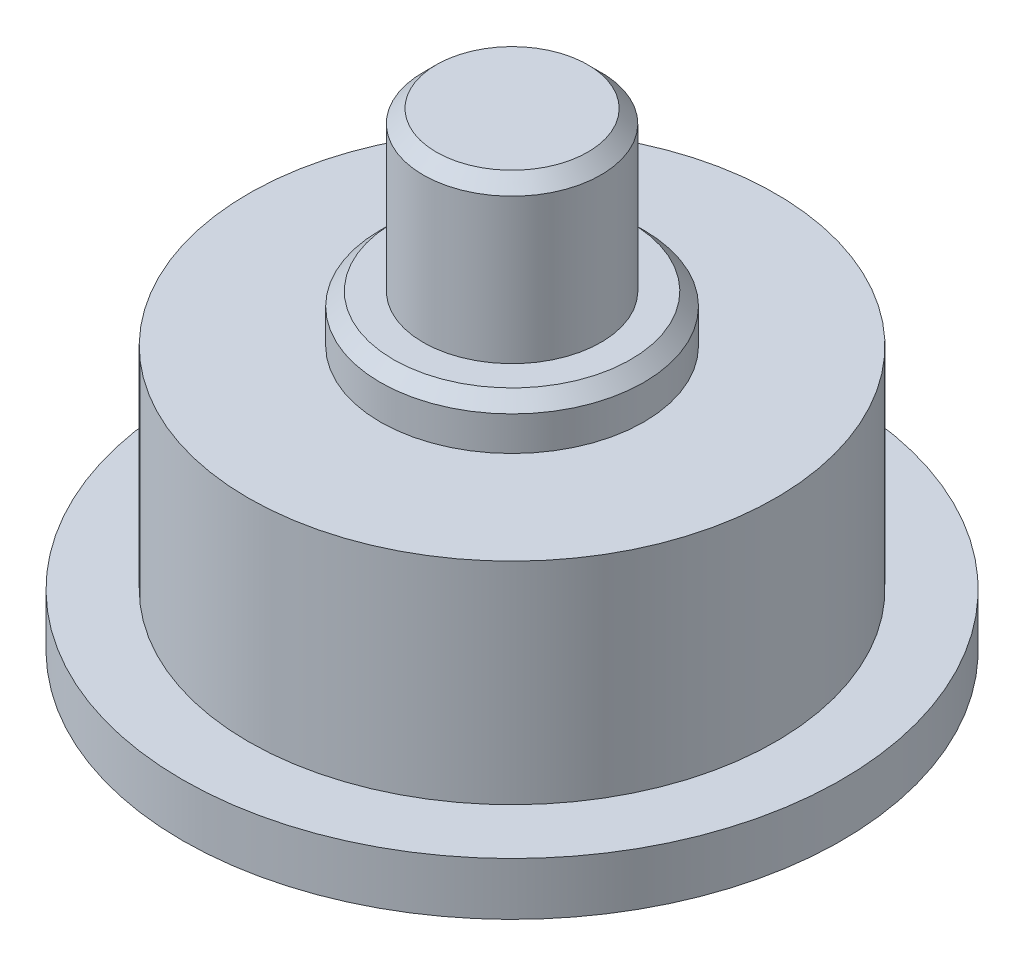
SolidWorks part; units mm, degrees
material "Q235B"
ref_plane "Front Plane" through (0, 0, 0) normal (0, 0, 1) x (1, 0, 0)
ref_plane "Top Plane" through (0, 0, 0) normal (0, 1, 0) x (1, 0, 0)
ref_plane "Right Plane" through (0, 0, 0) normal (1, 0, 0) x (0, 0, -1)
sketch "Sketch1" plane through (0, 0, 0) normal (0, 0, 1) x (1, 0, 0)
  line L0 (24.234, -52.0306) -> (24.234, -74.1987) construction
  line L2 (-3.466, -62.3306) -> (36.234, -62.3306) construction
  line L3 (20.8612, -54.5306) -> (24.234, -54.5306)
  line L6 (19.234, -62.3306) -> (14.234, -62.3306)
  line L9 (14.234, -62.3306) -> (14.234, -70.3306)
  line L10 (20.8612, -54.5306) -> (20.8612, -60.5306)
  line L11 (20.8612, -60.5306) -> (19.234, -60.5306)
  line L12 (19.234, -60.0306) -> (19.234, -62.3306) construction
  line L13 (19.234, -60.5306) -> (19.234, -62.3306)
  line L19 (36.234, -60.0306) -> (-3.466, -60.0306) construction
  line L23 (14.234, -70.3306) -> (11.734, -70.3306)
  line L24 (11.734, -70.3306) -> (11.734, -72.3306)
  line L25 (11.734, -72.3306) -> (24.234, -72.3306)
  line L28 (31.234, -52.0306) -> (17.234, -52.0306) construction
  line L29 (24.234, -72.3306) -> (24.234, -54.5306)
  dimension "D1" = 0.5
  dimension "D2" = 20
  dimension "D3" = 6
  dimension "D4" = 25
  dimension "D5" = 8
  dimension "D6" = 6.7456
  dimension "D7" = 2
revolve "Revolve8" add sketch "Sketch1" angle 360 about L0
chamfer "Chamfer1" distance 0.5 angle 45 2 edges at (24.234, -60.5306, 5) (24.234, -54.5306, 3.3728)
